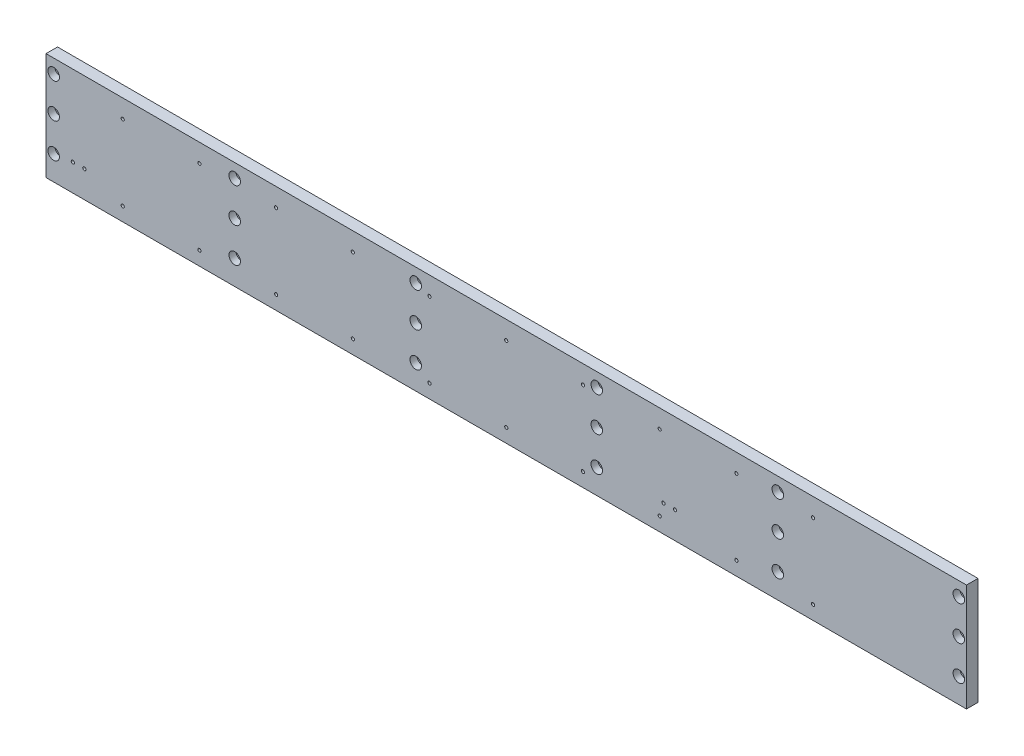
SolidWorks part; units mm, degrees
ref_plane "前视基准面" through (0, 0, 0) normal (0, 0, 1) x (1, 0, 0)
ref_plane "上视基准面" through (0, 0, 0) normal (0, 1, 0) x (1, 0, 0)
ref_plane "右视基准面" through (0, 0, 0) normal (1, 0, 0) x (0, 0, -1)
sketch "草图1" plane through (0, 0, 0) normal (0, 0, 1) x (1, 0, 0)
  line L1 (600, -70) -> (-600, -70)
  line L2 (600, -70) -> (600, 70)
  line L3 (600, 70) -> (-600, 70)
  line L4 (-600, -70) -> (-600, 70)
  line L5 (600, -70) -> (-600, 70) construction
  line L6 (600, 70) -> (-600, -70) construction
  point P0 (0, 0)
  dimension "D1" = 1200
  dimension "D2" = 140
extrude "凸台-拉伸1" add sketch "草图1" along normal mid plane 15
hole_wizard "M6 螺纹孔1" positions "3D草图1" profile "草图3" tap size "M6" standard "GB"
sketch3d "3D草图1"
  line L0 (-600, -70, 7.5) -> (-600, -70, -7.5) construction
  line L1 (-600, -70, -7.5) -> (600, -70, -7.5) construction
  point P0 (-590, -70, 0)
  dimension "D1" = 10
  dimension "D2" = 7.5
cosmetic thread "孔螺蚊线1" parameters "D1"=15, "D2"=6
sketch "草图3" plane through (-590, -70, 0) normal (1, 0, 0) x (0, 0, -1)
  line L0 (0, 0) -> (0, 20.0022)
  line L1 (0, 20.0022) -> (2.5, 18.5)
  line L2 (2.5, 18.5) -> (2.5, 0)
  line L5 (2.5, 0) -> (0, 0)
  line L10 (0, 20.0022) -> (-2.5, 18.5) construction
  line L11 (0, -6.35) -> (0, 107.95) construction
  dimension "螺纹孔钻头直径" = 5
  dimension "螺纹孔钻头深度" = 18.5
  dimension "导头角度" = 118
pattern_linear "阵列(线性)1" count 6 spacing 236 along (1, 0, 0) of "M6 螺纹孔1"
hole_wizard "打孔尺寸(%根据)内六角圆柱头螺钉的类型1" positions "草图6" profile "草图5" counterbore size "M8" standard "GB" end condition through all
sketch "草图6" plane through (0, 0, 7.5) normal (0, 0, 1) x (1, 0, 0)
  line L0 (-600, 70) -> (-600, -70) construction
  line L1 (-600, -70) -> (600, -70) construction
  point P0 (-590, 52)
  point P2 (-590, 7)
  point P4 (-590, -38)
  dimension "D1" = 10
  dimension "D2" = 32
  dimension "D3" = 45
  dimension "D4" = 45
sketch "草图5" plane through (-590, 52, 7.5) normal (1, 0, 0) x (0, -1, 0)
  line L0 (0, 0) -> (0, 15)
  line L1 (0, 15) -> (4.5, 15)
  line L3 (4.5, 15) -> (4.5, 9)
  line L4 (4.5, 9) -> (7.5, 9)
  line L5 (7.5, 9) -> (7.5, 0)
  line L7 (7.5, 0) -> (0, 0)
  line L11 (0, -6.35) -> (0, 107.95) construction
  dimension "通孔孔直径" = 9
  dimension "通孔孔深度" = 15
  dimension "柱形沉头孔直径" = 15
  dimension "柱形沉头孔深度" = 9
pattern_linear "阵列(线性)2" count 6 spacing 236 along (1, 0, 0) of "打孔尺寸(%根据)内六角圆柱头螺钉的类型1"
hole_wizard "M5 螺纹孔1" positions "草图10" profile "草图9" tap size "M5" standard "GB" end condition through all
sketch "草图10" plane through (0, 0, -7.5) normal (0, 0, -1) x (-1, 0, 0)
  line L0 (600, -70) -> (-600, -70) construction
  line L1 (600, 70) -> (600, -70) construction
  point P0 (550, -35)
  point P2 (565, -35)
  dimension "D1" = 35
  dimension "D2" = 35
  dimension "D3" = 15
cosmetic thread "孔螺蚊线2" parameters "D2"=5
cosmetic thread "孔螺蚊线3" parameters "D2"=5
sketch "草图9" plane through (-550, -35, -7.5) normal (1, 0, 0) x (0, 1, 0)
  line L0 (0, 0) -> (0, 15)
  line L1 (0, 15) -> (2.1, 15)
  line L2 (2.1, 15) -> (2.1, 0)
  line L5 (2.1, 0) -> (0, 0)
  line L11 (0, -6.35) -> (0, 107.95) construction
  dimension "通孔螺纹孔钻头直径" = 4.2
  dimension "通孔螺纹孔钻头深度" = 15
pattern_linear "阵列(线性)3" count 2 spacing 770 along (1, 0, 0) of "M5 螺纹孔1"
hole_wizard "M5 螺纹孔2" positions "草图12" profile "草图11" tap size "M5" standard "GB" end condition through all
sketch "草图12" plane through (0, 0, 7.5) normal (0, 0, 1) x (1, 0, 0)
  line L0 (600, 70) -> (-600, 70) construction
  line L1 (-600, 70) -> (-600, -70) construction
  point P0 (-500, 46)
  point P2 (-500, -52)
  dimension "D1" = 98
  dimension "D2" = 24
  dimension "D3" = 100
sketch "草图11" plane through (-500, 46, 7.5) normal (1, 0, 0) x (0, -1, 0)
  line L0 (0, 0) -> (0, 15)
  line L1 (0, 15) -> (2.1, 15)
  line L2 (2.1, 15) -> (2.1, 0)
  line L5 (2.1, 0) -> (0, 0)
  line L11 (0, -6.35) -> (0, 107.95) construction
  dimension "通孔螺纹孔钻头直径" = 4.2
  dimension "通孔螺纹孔钻头深度" = 15
cosmetic thread "孔螺蚊线4" parameters "D2"=5
cosmetic thread "孔螺蚊线5" parameters "D2"=5
pattern_linear "阵列(线性)4" count 10 spacing 100 along (1, 0, 0) of "M5 螺纹孔2"
